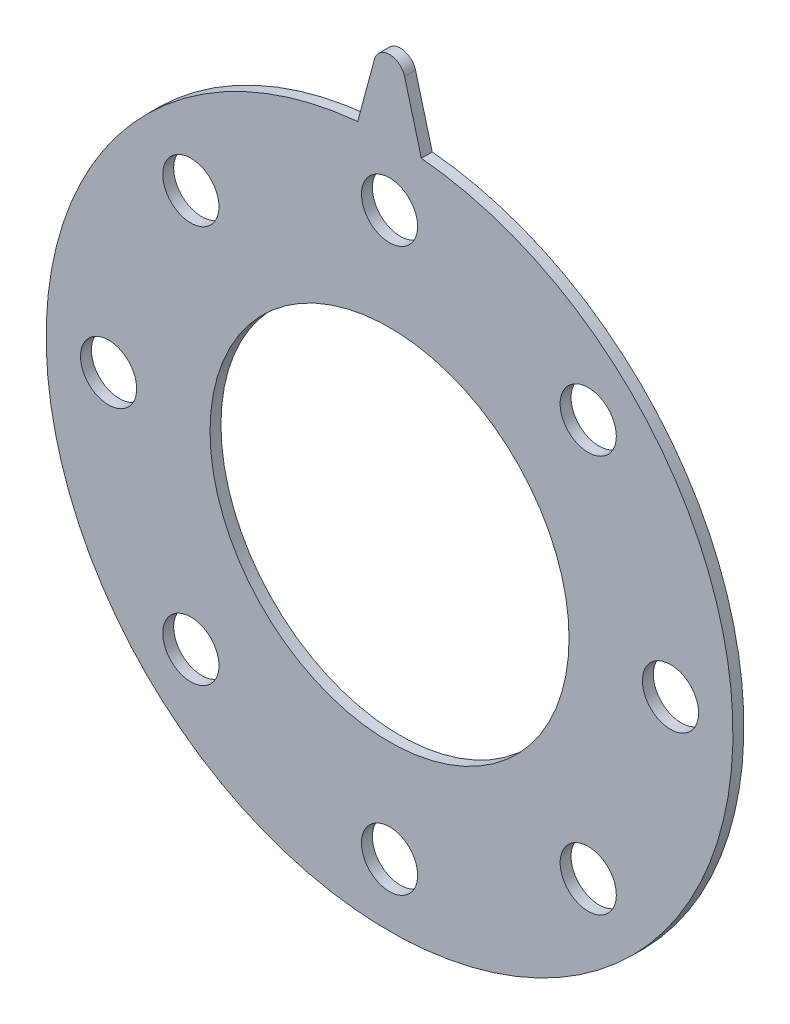
SolidWorks part; units mm, degrees
material "Rubber"
ref_plane "Front Plane" through (0, 0, 0) normal (0, 0, 1) x (1, 0, 0)
ref_plane "Top Plane" through (0, 0, 0) normal (0, 1, 0) x (1, 0, 0)
ref_plane "Right Plane" through (0, 0, 0) normal (1, 0, 0) x (0, 0, -1)
sketch "Sketch1" plane through (0, 0, 0) normal (0, 0, 1) x (1, 0, 0)
  line L0 (0, 128.233) -> (0, 110) construction
  line L1 (-4.8296, 129.5271) -> (-10.1886, 109.5271)
  line L2 (4.8296, 129.5271) -> (10.1886, 109.5271)
  arc A0 (-10.1886, 109.5271) -> (10.1886, 109.5271) centre (0, 0) ccw
  circle A1 centre (0, 0) radius 90 construction
  circle A2 centre (0, 0) radius 57.5
  circle A3 centre (0, 90) radius 9
  circle A4 centre (63.6396, 63.6396) radius 9
  circle A5 centre (90, 0) radius 9
  circle A6 centre (63.6396, -63.6396) radius 9
  circle A7 centre (0, -90) radius 9
  circle A8 centre (-63.6396, -63.6396) radius 9
  circle A9 centre (-90, 0) radius 9
  circle A10 centre (-63.6396, 63.6396) radius 9
  arc A12 (-4.8296, 129.5271) -> (4.8296, 129.5271) centre (0, 128.233) cw
  dimension "D1" = 220
  dimension "D2" = 180
  dimension "D3" = 115
  dimension "D4" = 18
  dimension "D7" = 5
  dimension "D6" = 20
  dimension "D8" = 30
  dimension "D9" = 15
  dimension "D5" = 8
extrude "Boss-Extrude1" add sketch "Sketch1" along normal blind 3.5
